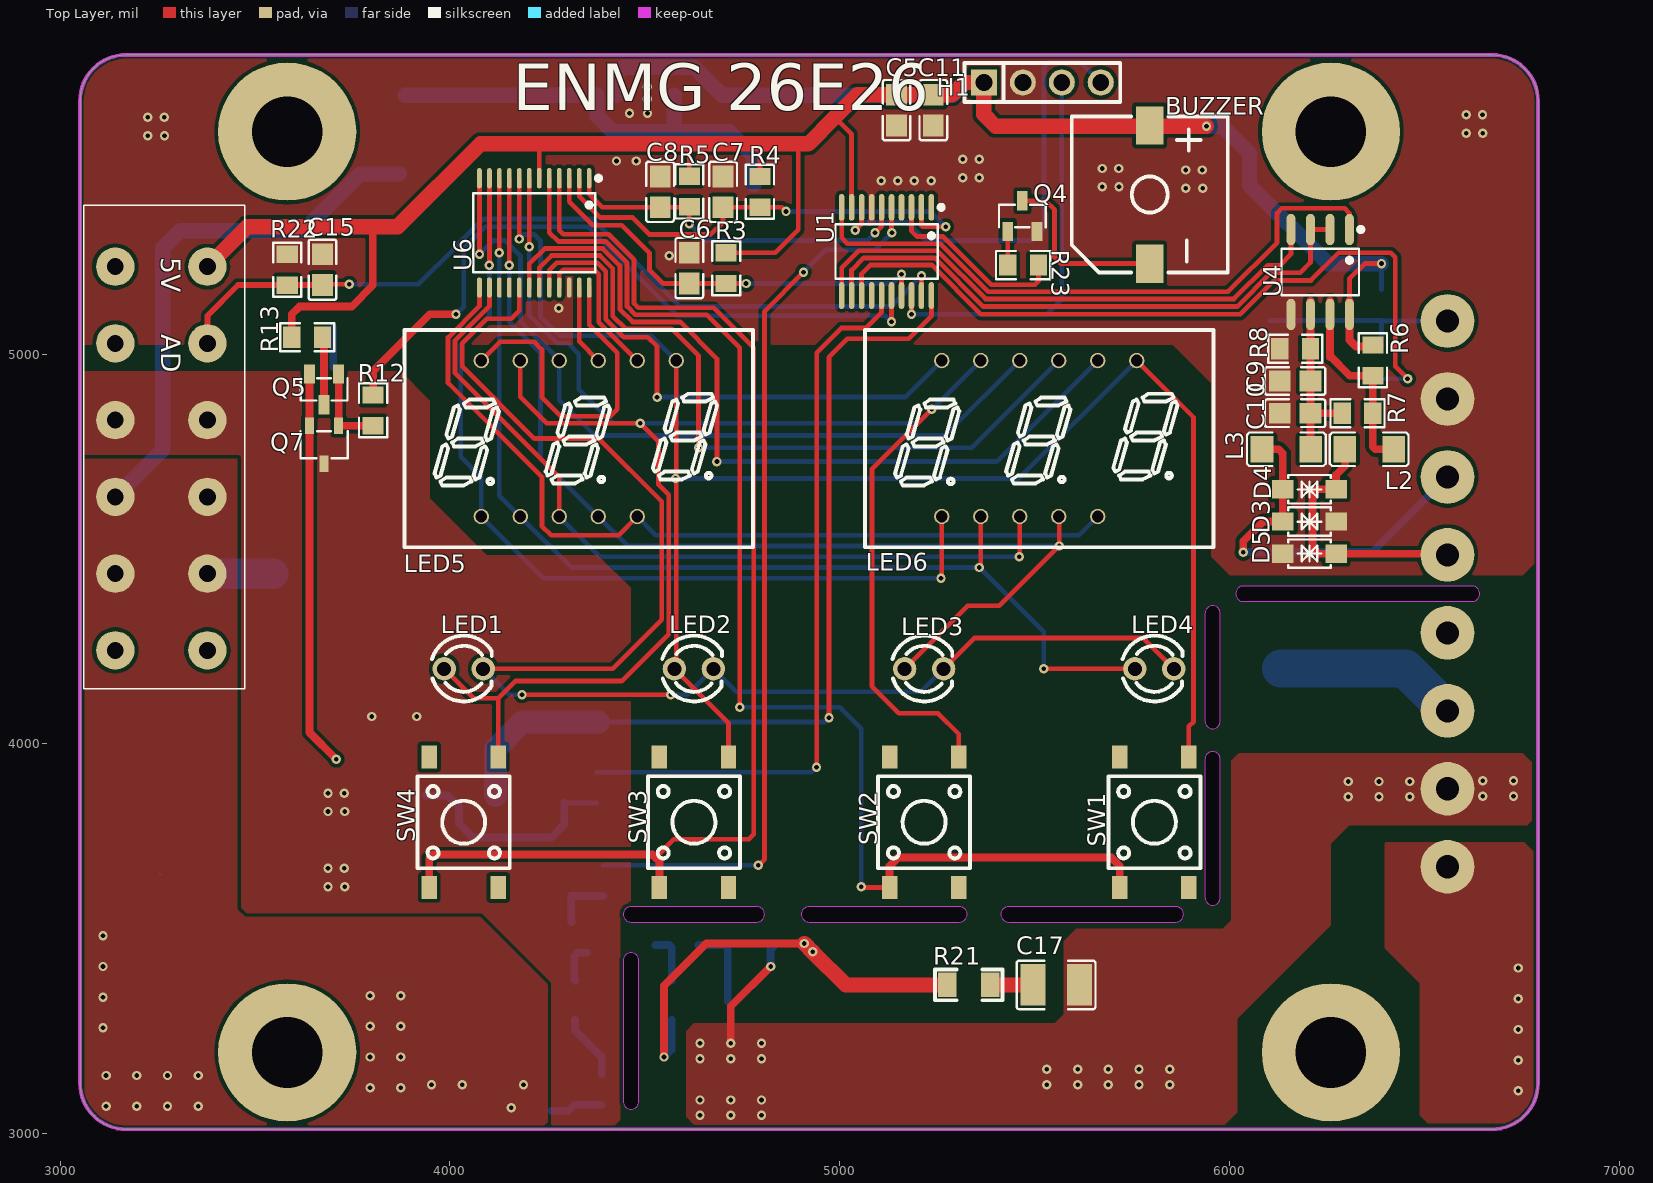
[diagram p0: Top Layer view]
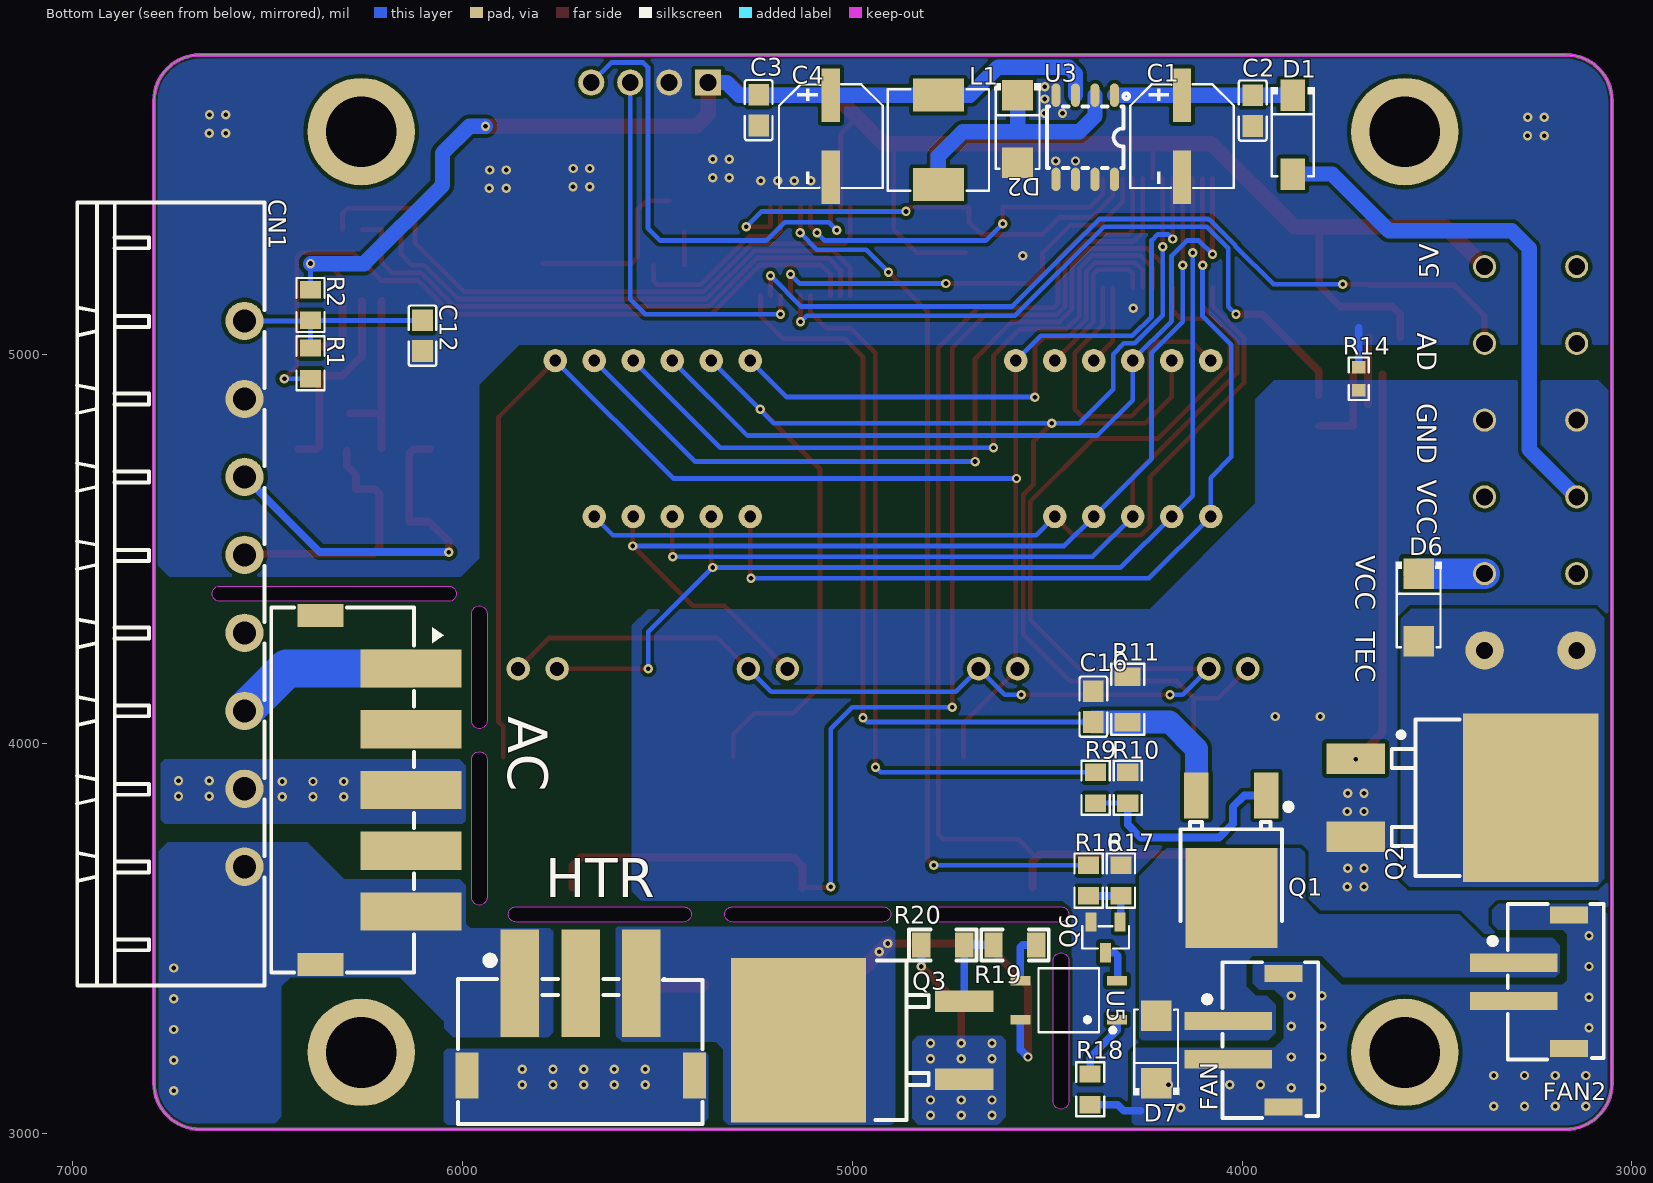
[diagram p1: Bottom Layer view, seen from below]
# Altium PCB MISC84275.PcbDoc (part 1 of 3)
Units mil, origin at the board's own origin, x right, y up, seen from the top; angles counter-clockwise.
Board outline 3740.1 x 2755.9 mil, 2 copper layers (Top Layer, Bottom Layer), stack 62.2 mil thick; 76 components, 62 nets, 275 pads, 150 vias.

## Layer stack, top to bottom
Top Solder Mask Layer: solder mask 0.4, Dk 3.3
Top Layer: signal copper 1.4
Dielectric1: surface 59.4, FR4, Dk 4.5
Bottom Layer: signal copper 1.4
Bottom Solder Mask Layer: solder mask 0.4, Dk 3.3

## Board outline
3169.3,5767.7 ccw(c3169.3,5649.6) 3051.2,5649.6 3051.2,3129.9 ccw(c3169.3,3129.9) 3169.3,3011.8 6673.2,3011.8 ccw(c6673.2,3129.9) 6791.3,3129.9 6791.3,5649.6 ccw(c6673.2,5649.6) 6673.2,5767.7
cut-out: 5956.7,3980.3 ccw(c5956.7,3960.6) 5937,3960.6 5937,3606.3 ccw(c5956.7,3606.3) 5956.7,3586.6 ccw(c5956.7,3606.3) 5976.4,3606.3 5976.4,3960.6 ccw(c5956.7,3960.6) 5956.7,3980.3
cut-out: 5413.4,3563 ccw(c5433.1,3563) 5433.1,3543.3 5862.2,3543.3 ccw(c5862.2,3563) 5881.9,3563 ccw(c5862.2,3563) 5862.2,3582.7 5433.1,3582.7 ccw(c5433.1,3563) 5413.4,3563
cut-out: 4901.6,3563 ccw(c4921.3,3563) 4921.3,3543.3 5307.1,3543.3 ccw(c5307.1,3563) 5326.8,3563 ccw(c5307.1,3563) 5307.1,3582.7 4921.3,3582.7 ccw(c4921.3,3563) 4901.6,3563
cut-out: 4444.9,3563 ccw(c4464.6,3563) 4464.6,3543.3 4787.4,3543.3 ccw(c4787.4,3563) 4807.1,3563 ccw(c4787.4,3563) 4787.4,3582.7 4464.6,3582.7 ccw(c4464.6,3563) 4444.9,3563
cut-out: 4464.6,3464.6 ccw(c4464.6,3444.9) 4444.9,3444.9 4444.9,3082.7 ccw(c4464.6,3082.7) 4464.6,3063 ccw(c4464.6,3082.7) 4484.3,3082.7 4484.3,3444.9 ccw(c4464.6,3444.9) 4464.6,3464.6
cut-out: 6015.7,4385.4 ccw(c6035.4,4385.4) 6035.4,4365.8 6622,4365.8 ccw(c6622,4385.4) 6641.7,4385.4 ccw(c6622,4385.4) 6622,4405.1 6035.4,4405.1 ccw(c6035.4,4385.4) 6015.7,4385.4
cut-out: 5956.7,4354.3 ccw(c5956.7,4334.6) 5937,4334.6 5937,4059.1 ccw(c5956.7,4059.1) 5956.7,4039.4 ccw(c5956.7,4059.1) 5976.4,4059.1 5976.4,4334.6 ccw(c5956.7,4334.6) 5956.7,4354.3

## Design rules (kind name [scope] priority, off if disabled: settings)
BoardOutlineClearance copperThickness1oz [All] p0: genericclearance=10 ignorepadtopadclearanceinfootprint=FALSE except(0: Arc-SplitContinuation Track-SplitContinuation SMDPad-SplitContinuation THPad-SplitContinuation Via-SplitContinuation Fill-SplitContinuation Poly-SplitContinuation Region-SplitContinuation Text-SplitContinuation)
BoardOutlineClearance copperThickness2oz [All] p0: genericclearance=10 ignorepadtopadclearanceinfootprint=FALSE except(0: Arc-SplitContinuation Track-SplitContinuation SMDPad-SplitContinuation THPad-SplitContinuation Via-SplitContinuation Fill-SplitContinuation Poly-SplitContinuation Region-SplitContinuation Text-SplitContinuation)
BoardOutlineClearance Plane_innerPlane [All] p0: genericclearance=10 ignorepadtopadclearanceinfootprint=FALSE except(0: Arc-SplitContinuation Track-SplitContinuation SMDPad-SplitContinuation THPad-SplitContinuation Via-SplitContinuation Fill-SplitContinuation Poly-SplitContinuation Region-SplitContinuation Text-SplitContinuation)
BoardOutlineClearance Copper_copperRegion [All] p0: genericclearance=10 ignorepadtopadclearanceinfootprint=FALSE except(0: Arc-SplitContinuation Track-SplitContinuation SMDPad-SplitContinuation THPad-SplitContinuation Via-SplitContinuation Fill-SplitContinuation Poly-SplitContinuation Region-SplitContinuation Text-SplitContinuation)
BoardOutlineClearance otherClearance [All] p0: genericclearance=10 ignorepadtopadclearanceinfootprint=FALSE except(0: Arc-SplitContinuation Track-SplitContinuation SMDPad-SplitContinuation THPad-SplitContinuation Via-SplitContinuation Fill-SplitContinuation Poly-SplitContinuation Region-SplitContinuation Text-SplitContinuation)
Clearance copperThickness1oz [All] p1: gap=7 ignorepadtopadclearanceinfootprint=FALSE
Clearance copperThickness2oz [All] p1: gap=7 ignorepadtopadclearanceinfootprint=FALSE
Clearance Plane_innerPlane [All] p1: gap=7 ignorepadtopadclearanceinfootprint=FALSE
Clearance Copper_copperRegion [All] p1: gap=7 ignorepadtopadclearanceinfootprint=FALSE
Clearance otherClearance [All] p1: gap=7 ignorepadtopadclearanceinfootprint=FALSE
DiffPairsRouting differentialPair [All] p1: maxuncoupledlength=10 minlimit=6 maxlimit=Infinity mostfreqgap=6 toplayer_minwidth=5 toplayer_prefwidth=10 toplayer_maxwidth=100 bottomlayer_minwidth=5 bottomlayer_prefwidth=10 bottomlayer_maxwidth=100
PasteMaskExpansion pasteMaskExpansion [All] p1: expansion=0
PlaneConnect innerPlane [All] p1: planeconnectstyle=Relief reliefexpansion=20 reliefentries=4 reliefconductorwidth=10 reliefairgap=10
PolygonConnect copperRegion [All] p1: connectstyle=Direct reliefentries=4 reliefconductorwidth=10 polygonreliefangle="90 Angle" airgapwidth=10
RoutingVias viaSize [All] p1: viastyle="Through Hole" holewidth=12.0078 minholewidth=11.811 maxholewidth=248.0314 width=12.0078 minwidth=11.811 maxwidth=248.0314
SolderMaskExpansion solderMaskExpansion [IsVia] p1: useseparateexpansions=TRUE expansion=-1000 expansionbottom=-1000
SolderMaskExpansion solderMaskExpansion [All] p2: useseparateexpansions=TRUE expansion=2 expansionbottom=2
Width copperThickness1oz [All] p1: maxlimit=100 minlimit=5 preferedwidth=10
Width copperThickness2oz [All] p1: maxlimit=100 minlimit=8 preferedwidth=10
Width trackWidth1 [All] p1: maxlimit=100 minlimit=5 preferedwidth=30

## Components (designator, comment, footprint, x,y, rotation, side; value= is the part's Value field where it differs from the comment)
AC "BX-VH3.96-5PLT" CONN-SMD_5P-P3.96_BX-VH3.96-5PLT 6248,3881.9 r270 bottom
BUZZER "2.7kHz" BUZ-SMD_L9.6-W9.6-LS10.0-R 5795.3,5409.4 r90 top
C1 "220uF" CAP-SMD_BD6.3-L6.6-W6.6-FD 4154.1,5559.1 r270 bottom
C2 "100nF" C0805#1 3972.7,5624.8 r270 bottom
C3 "100nF" C0805#1 5240.2,5626 r90 bottom
C4 "220uF" CAP-SMD_BD6.3-L6.6-W6.6-FD 5054.9,5559.1 r270 bottom
C5 "100nF" C0805#1 5145.7,5626 r270 top
C6 "100pF" C0805#2 4614.2,5220.5 r270 top
C7 "100pF" C0805#3 4700.8,5416.3 r270 top
C8 "100pF" C0805#3 4539.4,5416.3 r270 top
C9 "100nF" C0805#1 6168.2,4931.2 r0 top
C10 "100nF" C0805#1 6168.2,4848.5 r0 top
C11 "100nF" C0805#1 5240.2,5626 r90 top
C12 "1nF" C0805#3 6102.4,5047.2 r270 bottom
C15 "100nF" C0805#3 3673.2,5216.5 r270 top
C16 "100nF" C0805#2 4381.7,4095.7 r270 bottom
C17 "10nF" C1210 5555.1,3381.9 r180 top
CN1 "KF2EDGRM-5.08-8P" CONN-TH_8P-P5.08_KF2EDGRM-5.08-8P 6559.1,4385.1 r270 bottom
D1 "M7" SMA_L4.4-W2.8-LS5.4-RD 3870.1,5563 r270 bottom
D2 "SS34" SMA_L4.3-W2.6-LS5.2-RD 4576,5577.6 r270 bottom
D3 "SMF36CA" SOD-123_L2.7-W1.8-LS3.7-BI 6205,4570.8 r0 top
D4 "SMF36CA" SOD-123_L2.7-W1.8-LS3.7-BI 6205,4653.5 r0 top
D5 "SMF36CA" SOD-123_L2.7-W1.8-LS3.7-BI 6205,4488.1 r180 top
D6 "SS34" SMA_L4.3-W2.6-LS5.2-RD 3547.2,4350.4 r270 bottom
D7 "SS34" SMA_L4.3-W2.6-LS5.2-RD 4220.5,3216.5 r90 bottom
FAN "XH2.54-2P vertical SMD" CONN-SMD_2P_A2501WV-S#1 3964.6,3240.2 r90 bottom
FAN2 "XH2.54-2P vertical SMD" CONN-SMD_2P_A2501WV-S#2 3232.3,3389.8 r90 bottom
H1 "PZ254V-11-04P" HDR-TH_4P-P2.54-V-M 5519.7,5696.9 r0 top
HTR "VH3.96-3P" CONN-SMD_3P-P3.96_HCTL_HC-VH-3ALT 5696.9,3267.7 r180 bottom
L1 "68uH" IND-SMD_L7.1-W6.6_H5.0 4779.1,5549.5 r270 bottom
L2 "22uH" L1206 6358.3,4755.9 r180 top
L3 "22uH" L1206 6145.7,4755.9 r180 top
LED1 "3mmFIR" LED-TH_BD3.0-P2.54-FD 4035.4,4192.9 r0 top
LED2 "3mmFIR" LED-TH_BD3.0-P2.54-FD 4626,4192.9 r0 top
LED3 "3mmFIR" LED-TH_BD3.0-P2.54-FD 5216.5,4192.9 r0 top
LED4 "3mmFIR" LED-TH_BD3.0-P2.54-FD 5807.1,4192.9 r0 top
LED5 "SP420361N" LED-SEG-TH_SP420361N 4330.7,4783.5 r270 top
LED6 "SP420361N" LED-SEG-TH_SP420361N 5511.8,4783.5 r270 top
Q1 "NCE0140K2-VB" TO-252-3_L6.6-W6.1-P4.58-LS10.1-BR 4027.6,3736.2 r90 bottom
Q2 "HYG025N06LS1B" TO-263-2_L10.2-W8.7-P5.08-LS15.1-BR 3484.3,3862.2 r0 bottom
Q3 "BTA216B-600D-JSM" TO-263-3_L10.2-W9.2-P5.08-LS15.4-BR 4925.2,3240.2 r180 bottom
Q4 "SS8050(RANGE:200-350)" SOT-23-3_L2.9-W1.3-P1.90-LS2.4-BR#1 5468.5,5354.3 r270 top
Q5 "SS8050(RANGE:200-350)" SOT-23-3_L2.9-W1.3-P1.90-LS2.4-BR#2 3677.2,4909.4 r90 top
Q6 "SS8050(RANGE:200-350)" SOT-23-3_L2.9-W1.3-P1.90-LS2.4-BR#2 4350.4,3503.9 r90 bottom
Q7 "LBC807-25LT1G" SOT-23-3_L2.9-W1.6-P1.90-LS2.8-BR 3677.2,4767.7 r90 top
R1 "1kΩ" R0805#1 6389.8,4976.4 r90 bottom
R2 "1kΩ" R0805#2 6389.8,5126 r90 bottom
R3 "10kΩ" R0805#1 4708.7,5220.5 r90 top
R4 "10kΩ" R0805#3 4795.3,5416.3 r90 top
R5 "10kΩ" R0805#3 4614.2,5417.3 r90 top
R6 "47kΩ" R0805#2 6367.6,4984.2 r90 top
R7 "12kΩ" R0805#2 6328.2,4848.5 r0 top
R8 "47kΩ" R0805#2 6168.2,5013.9 r0 top
R9 "10K" R0805#2 4376,3887.8 r270 bottom
R10 "10kΩ" R0805#2 4293.3,3887.8 r270 bottom
R11 "1Ω" R1206 4293.6,4114.5 r270 bottom
R12 "1kΩ" R0805#2 3803.1,4855.7 r270 top
R13 "47Ω" R0805#3 3633.9,5043.3 r180 top
R14 "10K" R0603 3700.8,4937 r90 bottom
R16 "1kΩ" R0805#2 4393.7,3649.6 r270 bottom
R17 "10kΩ" R0805#2 4311,3649.6 r90 bottom
R18 "2.2kΩ" R0805#3 4389.8,3114.2 r270 bottom
R19 "51Ω" R0204 4582.7,3484.3 r0 bottom
R20 "150Ω" R0204 4767.7,3484.3 r0 bottom
R21 "120Ω" R0204 5330.7,3381.9 r180 top
R22 "10kΩ" R0805#1 3582.7,5216.5 r270 top
R23 "1kΩ" R0805#3 5470.5,5228.3 r180 top
SW1 "1TS005F-2500-5001" SW-SMD_4P-L6.0-W6.0-P4.50-LS9.0-H2.5#1 5807.1,3799.2 r90 top
SW2 "1TS005F-2500-5001" SW-SMD_4P-L6.0-W6.0-P4.50-LS9.0-H2.5#2 5216.5,3799.2 r90 top
SW3 "1TS005F-2500-5001" SW-SMD_4P-L6.0-W6.0-P4.50-LS9.0-H2.5#1 4626,3799.2 r90 top
SW4 "1TS005F-2500-5001" SW-SMD_4P-L6.0-W6.0-P4.50-LS9.0-H2.5#2 4035.4,3799.2 r90 top
U1 "LCM08F003" TSSOP-20_L6.5-W4.4-P0.65-LS6.4-BL 5120.1,5263.5 r180 top
U3 "XL1509-5.0" SOIC-8_L4.9-W3.9-P1.27-LS6.0-TR 4402.5,5556.3 r180 bottom
U4 "MAX485ESA(UMW)" SOP-8_L5.0-W4.0-P1.27-LS6.0-BL 6232.6,5210.7 r180 top
U5 "ELM3083(TA)-V" SOP-4_L4.4-W4.0-P2.54-LS7.0-TL 4444.9,3342.5 r0 bottom
U6 "TM1668-SSOP24-TA2108" SSOP-24_L8.1-W5.3-P0.65-LS7.8-BL 4216.5,5311 r180 top

## Footprints (in the part's own frame and the unit in brackets; to place one, negate y for a bottom-side part, rotate by r counter-clockwise, add the part's x,y. Pads: shape width x height; smd on the part's side, far side on the other; paste and mask are expansions set on the pad)
BUZ-SMD_L9.6-W9.6-LS10.0-R [mil]
  rect 98.4x70.9 smd: 1(177.2,0) 2(-177.1,0)
  silkscreen extent -200,-200 200,200
C0805#1 [mil]
  rect 55.5x53.1 smd paste-3937 mask+2: 1(-39.4,0) 2(39.4,0)
  silkscreen extent -77,-36 77,36
C0805#2 [mil]
  rect 55.5x53.1 smd paste-3937 mask+2: 1(-39.3,0) 2(39.4,0)
  silkscreen extent -77,-36 77,36
C0805#3 [mil]
  rect 55.5x53.1 smd paste-3937 mask+2: 1(-39.4,0) 2(39.3,0)
  silkscreen extent -77,-36 77,36
C1210 [mil]
  rect 64.4x106.3 smd paste-3937 mask+2: 1(-59.8,0) 2(59.7,0)
  silkscreen extent -101,-62 101,62
CAP-SMD_BD6.3-L6.6-W6.6-FD [mil]
  rect 137.8x47.2 smd: 1(-105.1,0) 2(105.2,0)
  silkscreen extent -133,-133 133,133
CONN-SMD_2P_A2501WV-S#1 [mil]
  rect 47.2x224.4 smd paste+0 mask+2: 1(49.2,70.8) 2(-49.3,70.8)
  rect 43.3x98.4 smd paste+0 mask+2: 3(-171.3,-70.9) 4(171.2,-70.9)
  silkscreen extent -199,-160 200,133
CONN-SMD_2P_A2501WV-S#2 [mil]
  rect 47.2x224.4 smd paste+0 mask+2: 1(49.2,70.8) 2(-49.2,70.8)
  rect 43.3x98.4 smd paste+0 mask+2: 3(-171.3,-70.9) 4(171.2,-70.9)
  silkscreen extent -199,-160 200,133
CONN-SMD_3P-P3.96_HCTL_HC-VH-3ALT [mil]
  rect 98.4x275.6 smd paste+0 mask+2: 1(-155.9,118.1) 2(0.1,118.1) 3(156,118.1)
  rect 59.1x118.1 smd paste+0 mask+2: 4(291.8,-118.1) 5(-291.7,-118.1)
  silkscreen extent -314,-242 313,187
CONN-SMD_5P-P3.96_BX-VH3.96-5PLT [mil]
  rect 98.4x259.8 smd paste+0 mask+2: 1(-311.8,116.1) 2(-155.9,116.1) 3(0,116.1) 4(155.9,116.1) 5(311.8,116.1)
  rect 59.1x118.1 smd paste+0 mask+2: 7(447.6,-116.2) 8(-447.6,-116.2)
  silkscreen extent -468,-243 468,201
CONN-TH_8P-P5.08_KF2EDGRM-5.08-8P [mil]
  round 98.4 / inner round 98.4 / far side round 137.8 hole 59.1: 1(-700,0) 2(-500,0) 3(-300,0) 4(-100,0) 5(100,0) 6(300,0) 7(500,0) 8(700,0)
  silkscreen extent -1004,-430 1004,51
HDR-TH_4P-P2.54-V-M [mil]
  rect 66.9x66.9 hole 43.3: 1(-150,0)
  round 66.9 hole 43.3: 2(-50,0) 3(50,0) 4(150,0)
  silkscreen extent -200,-50 200,50
IND-SMD_L7.1-W6.6_H5.0 [mil]
  rect 84.6x130.7 smd: 1(-114.7,0) 2(114.7,0)
  silkscreen extent -130,-130 130,130
L1206 [mil]
  rect 58.5x68 smd paste-3937 mask+2: 1(-62.7,0) 2(62.7,0)
  silkscreen extent -101,-43 101,43
LED-SEG-TH_SP420361N [mil]
  round 39.4 / inner round 39.4 / far side round 60 hole 30: 1(200,-250) 2(200,-150) 3(200,-50) 4(200,50) 5(200,150) 7(-200,250) 8(-200,150) 9(-200,50) 10(-200,-50) 11(-200,-150) 12(-200,-250)
  silkscreen extent -279,-447 279,447
LED-TH_BD3.0-P2.54-FD [mil]
  round 60 hole 36: 1(-50,0) 2(50,0)
  silkscreen extent -81,-84 72,85
R0204 [mil]
  rect 47.2x63 smd paste+0 mask+2: 1(-55.1,0) 2(55.1,0)
  silkscreen extent -87,-39 87,39
R0603 [mil]
  rect 31.8x34 smd paste-3937 mask+2: 1(-29.7,0) 2(29.7,0)
  silkscreen extent -54,-26 54,26
R0805#1 [mil]
  rect 44.6x54.2 smd paste-3937 mask+2: 1(-39.4,0) 2(39.3,0)
  silkscreen extent -69,-36 69,36
R0805#2 [mil]
  rect 44.6x54.2 smd paste-3937 mask+2: 1(-39.4,0) 2(39.4,0)
  silkscreen extent -69,-36 69,36
R0805#3 [mil]
  rect 44.6x54.2 smd paste-3937 mask+2: 1(-39.3,0) 2(39.4,0)
  silkscreen extent -69,-36 69,36
R1206 [mil]
  rect 47.5x67 smd paste-3937 mask+2: 1(-58.2,0) 2(58.2,0)
  silkscreen extent -91,-42 91,43
SMA_L4.3-W2.6-LS5.2-RD [mil]
  rect 78.7x78.7 smd: 1(-86.6,0) 2(86.6,0)
  silkscreen extent -117,-59 103,59
SMA_L4.4-W2.8-LS5.4-RD [mil]
  rect 80.6x63.8 smd: 1(-101,0) 2(101,0)
  silkscreen extent -121,-57 106,57
SOD-123_L2.7-W1.8-LS3.7-BI [mil]
  rect 55.1x47.2 smd: 1(-68.3,0) 2(68.3,0)
  silkscreen extent -54,-36 54,36
SOIC-8_L4.9-W3.9-P1.27-LS6.0-TR [mil]
  oval 23.6x59.8 smd: 1(75,107.9) 2(25,107.9) 3(-25,107.9) 4(-75,107.9) 5(-75,-107.9) 6(-25,-107.9) 7(25,-107.9) 8(75,-107.9)
  silkscreen extent -99,-79 113,112
SOP-4_L4.4-W4.0-P2.54-LS7.0-TL [mil]
  rect 51.2x23.4 smd: 1(-124,50) 2(-124,-50) 3(124,-50) 4(124,50)
  silkscreen extent -119,-82 78,82
SOP-8_L5.0-W4.0-P1.27-LS6.0-BL [mil]
  oval 22.6x80.1 smd: 1(-75,-109) 2(-25,-109) 3(25,-109) 4(75,-109) 5(75,108.9) 6(25,108.9) 7(-25,108.9) 8(-75,108.9)
  silkscreen extent -110,-115 100,60
SOT-23-3_L2.9-W1.3-P1.90-LS2.4-BR#1 [mil]
  rect 49.2x27.6 smd: 1(39.3,-37.4) 2(39.3,37.4) 3(-39.4,0)
  silkscreen extent -29,-60 29,60
SOT-23-3_L2.9-W1.3-P1.90-LS2.4-BR#2 [mil]
  rect 49.2x27.6 smd: 1(39.4,-37.4) 2(39.4,37.4) 3(-39.3,0)
  silkscreen extent -29,-60 29,60
SOT-23-3_L2.9-W1.6-P1.90-LS2.8-BR [mil]
  rect 42.1x23.6 smd: 1(48.6,-37.4) 2(48.6,37.4) 3(-48.6,0)
  silkscreen extent -35,-60 35,60
SSOP-24_L8.1-W5.3-P0.65-LS7.8-BL [mil]
  oval 12.1x52.1 smd: 1(-140.8,-140.3) 2(-115.2,-140.3) 3(-89.6,-140.3) 4(-64,-140.3) 5(-38.4,-140.3) 6(-12.8,-140.3) 7(12.8,-140.3) 8(38.4,-140.3) 9(63.9,-140.3) 10(89.5,-140.3) 11(115.1,-140.3) 12(140.7,-140.3) 13(140.7,140.2) 14(115.1,140.2) 15(89.5,140.2) 16(63.9,140.2) 17(38.4,140.2) 18(12.8,140.2) 19(-12.8,140.2) 20(-38.4,140.2) 21(-64,140.2) 22(-89.6,140.2) 23(-115.2,140.2) 24(-140.8,140.2)
  silkscreen extent -171,-146 156,101
SW-SMD_4P-L6.0-W6.0-P4.50-LS9.0-H2.5#1 [mil]
  rect 59.1x39.4 smd: 1(-167.3,88.6) 2(167.3,88.6) 3(-167.3,-88.6) 4(167.3,-88.6)
  silkscreen extent -118,-118 118,118
SW-SMD_4P-L6.0-W6.0-P4.50-LS9.0-H2.5#2 [mil]
  rect 59.1x39.4 smd: 1(-167.3,88.5) 2(167.3,88.5) 3(-167.3,-88.6) 4(167.3,-88.6)
  silkscreen extent -118,-118 118,118
TO-252-3_L6.6-W6.1-P4.58-LS10.1-BR [mil]
  rect 118.1x63 smd: 1(131.6,-90) 2(131.6,89.9)
  rect 255.9x236.2 smd: 3(-131.6,0)
  silkscreen extent -190,-154 111,130
TO-263-2_L10.2-W8.7-P5.08-LS15.1-BR [mil]
  rect 150x78.7 smd: 1(224.5,-100) 3(224.5,100)
  rect 348x433.1 smd: 4(-224.6,0)
  silkscreen extent -42,-201 132,201
TO-263-3_L10.2-W9.2-P5.08-LS15.4-BR [mil]
  rect 149.6x55.1 smd: 1(212.6,-100) 3(212.6,100)
  rect 346.5x421.3 smd: 2(-212.6,0)
  silkscreen extent -15,-205 121,205
TSSOP-20_L6.5-W4.4-P0.65-LS6.4-BL [mil]
  oval 14.3x68.6 smd: 1(-115.2,-113) 2(-89.6,-113) 3(-64,-113) 4(-38.4,-113) 5(-12.8,-113) 6(12.8,-113) 7(38.4,-113) 8(64,-113) 9(89.6,-113) 10(115.2,-113) 11(115.2,113) 12(89.6,113) 13(64,113) 14(38.4,113) 15(12.8,113) 16(-12.8,113) 17(-38.4,113) 18(-64,113) 19(-89.6,113) 20(-115.2,113)
  silkscreen extent -146,-119 131,70

## Free pads (board coordinates)
  round 98.4 / inner round 51.2 / far side round 98.4 hole 43.3 paste+0 mask+4: 0(3141.7,4240.2) 0(3378,4240.2)
  round 98.4 / inner round 51.2 / far side round 59.1 hole 43.3 paste+0 mask+4: 0(3141.7,4437) 0(3141.7,4633.9) 0(3141.7,4830.7) 0(3141.7,5027.6) 0(3141.7,5224.4) 0(3378,4437) 0(3378,4633.9) 0(3378,4830.7) 0(3378,5027.6) 0(3378,5224.4)
  round 354.3 / inner round 196.9 / far side round 275.6 hole 181.1: 1(3582.7,5570.9) 2(6259.8,5570.9) 3(6259.8,3208.7) 4(3582.7,3208.7)

## Via types
v1: diameter 24, hole 12, Top Layer to Bottom Layer, 150 vias

## Nets (pads, with @x,y where several pads share a name; then routed paths per layer and width w, separated by ;. In a path a pad name is that pad's centre, name@x,y a point inside that pad or via, vN(x,y) a via of type N, cw(c..) or ccw(c..) an arc to the next point about the centre after c; other vN are vias at no path point)
1: LED5.12 U6.24 | length 868.1
  Top Layer w12.1: LED5.12@4080.7,4983.5 4128.7,5031.5 4216.5,5031.5 4236.2,5011.8 4236.2,4889.8 4285,4841 4411.8,4841 4429.1,4858.3 4429.1,5003 4357.3,5074.8 U6.24@4357.3,5170.8
2: LED5.9 U6.23 | length 207.6
  Top Layer w12.1: U6.23@4331.7,5170.8 4331.7,5032.5 LED5.9@4380.7,4983.5
3: LED5.8 U6.21 | length 407.6
  Top Layer w12.1: U6.21@4280.5,5170.8 4280.5,5205.7 4291.3,5216.5 4369.8,5216.5 4381.9,5204.4 4381.9,5082.3 LED5.8@4480.7,4983.5
4: LED6.12 U6.20 | length 1389.1
  Top Layer w12.1: U6.20@4254.9,5170.8 4254.9,5215.6 4274,5234.7 4377.6,5234.7 4400,5212.2 4400,5089.8 4446.5,5043.3 4507.9,5043.3 4531.5,5019.7 v1(4531.5,4889.8)
  Bottom Layer w12.1: v1(4531.5,4889.8) 5168.1,4889.8 LED6.12@5261.8,4983.5
5: LED6.9 U6.19 | length 1903.2
  Top Layer w12.1: U6.19@4229.3,5170.8 4229.3,5221.5 4260.7,5252.8 4385.1,5252.8 4418.1,5219.7 4418.1,5097.3 4450.9,5064.6 4569.3,5064.6 4637.8,4996.1 v1(4637.8,4759.8)
  Bottom Layer w12.1: v1(4637.8,4759.8) 5338.2,4759.8 LED6.9@5561.8,4983.5
6: LED6.8 U6.18 | length 2089
  Top Layer w12.1: U6.18@4203.7,5170.8 4203.7,5231.3 4243.4,5270.9 4392.6,5270.9 4436.3,5227.2 4436.3,5114.9 4468.5,5082.7 4590.6,5082.7 4685,4988.2 v1(4685,4724.4)
  Bottom Layer w12.1: v1(4685,4724.4) 5402.8,4724.4 LED6.8@5661.8,4983.5